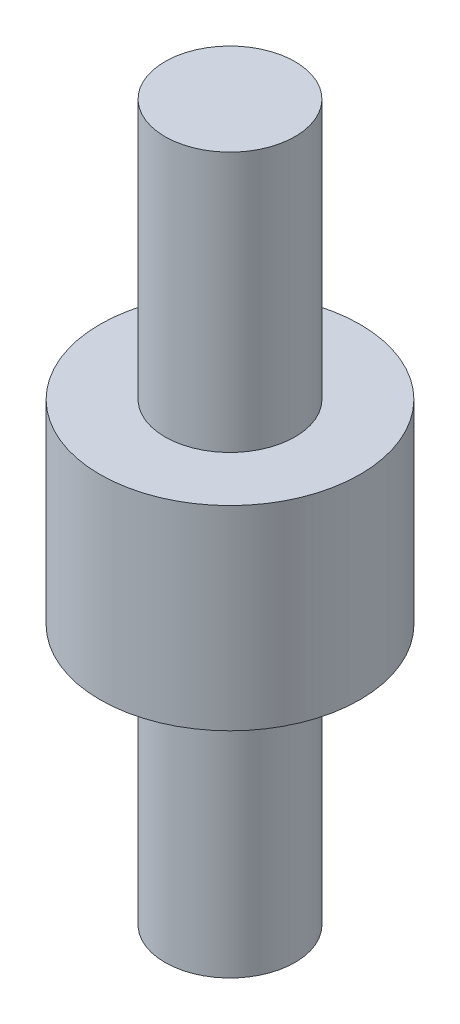
SolidWorks part; units mm, degrees
ref_plane "Front Plane" through (0, 0, 0) normal (0, 0, 1) x (1, 0, 0)
ref_plane "Top Plane" through (0, 0, 0) normal (0, 1, 0) x (1, 0, 0)
ref_plane "Right Plane" through (0, 0, 0) normal (1, 0, 0) x (0, 0, -1)
sketch "Sketch1" plane through (0, 0, 0) normal (1, 0, 0) x (0, 0, -1)
  line L0 (0, 189.9298) -> (0, -191.0006) construction
  line L1 (0, 55) -> (-10, 55)
  line L2 (-10, 55) -> (-10, 15)
  line L3 (-10, 15) -> (-20, 15)
  line L4 (-20, 15) -> (-20, -15)
  line L5 (-20, -15) -> (-10, -15)
  line L6 (-10, -15) -> (-10, -55)
  line L7 (-10, -55) -> (0, -55)
  line L8 (-62.7016, 0) -> (75.2789, 0) construction
  line L9 (0, 55) -> (0, -55)
  dimension "D1" = 30
  dimension "D2" = 10
  dimension "D3" = 20
  dimension "D4" = 40
revolve "Revolve1" add sketch "Sketch1" angle 360 about L0
ref_plane "Plane1" through (0, 0, -10) normal (0, 0, -1) x (-1, 0, 0)
sketch "Sketch2" plane through (0, 0, -10) normal (0, 0, -1) x (-1, 0, 0)
  line L0 (0, 154.7138) -> (0, 101.824) construction
  line L1 (0, 45) -> (0, 25) construction
  line L2 (2.5, 45) -> (2.5, 25)
  line L3 (-2.5, 45) -> (-2.5, 25)
  line L4 (10, 55) -> (-10, 55) construction
  arc A0 (2.5, 45) -> (-2.5, 45) centre (0, 45) ccw
  arc A1 (-2.5, 25) -> (2.5, 25) centre (0, 25) ccw
  point P5 (0, 35)
  dimension "D2" = 2.5
  dimension "D1" = 20
  dimension "D3" = 20
extrude "Cut-Extrude1" cut sketch "Sketch2" against normal blind 2.5
mirror "Mirror1" about plane through (0, 0, 0) normal (0, 1, 0) of "Cut-Extrude1"
